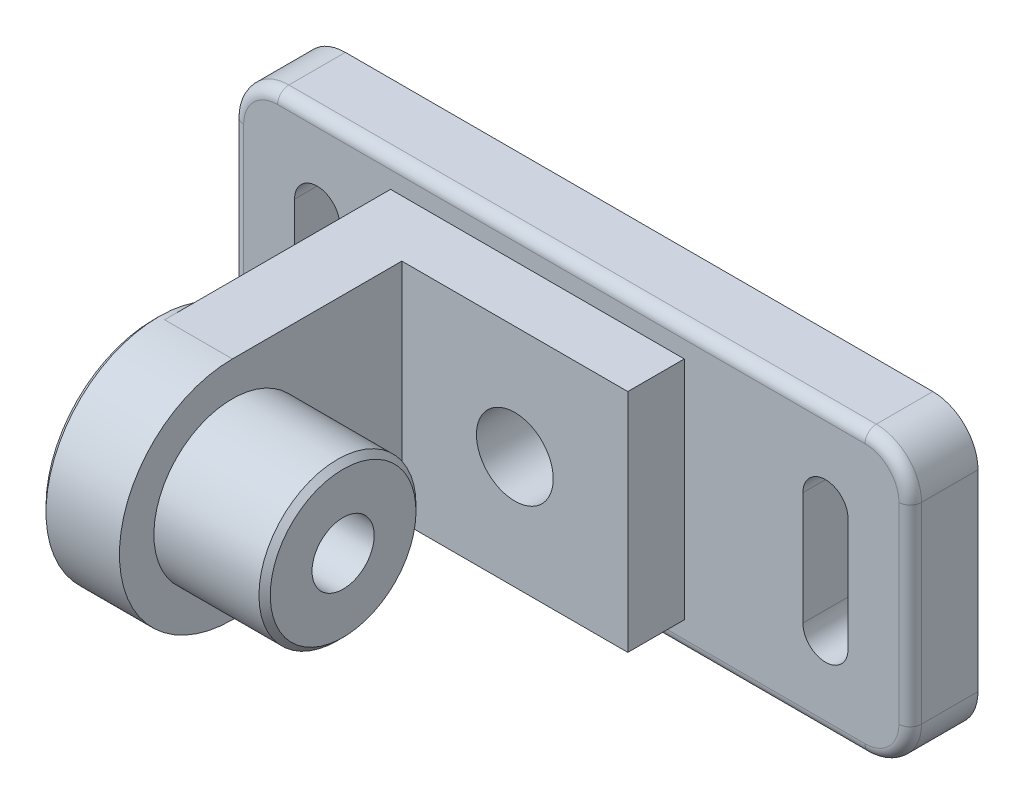
from build123d import *
from build123d.topology import SkipClean

# Parameters (mm, degrees)
SKETCH1_R               = 3.4
BOSS_EXTRUDE1_DEPTH     = 6
CHAMFER1_SIZE           = 1
SKETCH2_W               = 6
SKETCH2_H               = 20
BOSS_EXTRUDE2_DEPTH     = 30
CUT_EXTRUDE1_DEPTH      = 60.73483071
CUT_EXTRUDE1_DEPTH_BACK = 60.73483071
SKETCH3_R               = 2.75
SKETCH4_R               = 10
SKETCH4_R_2             = 2.75
BOSS_EXTRUDE3_DEPTH     = 1
CHAMFER2_SIZE           = 0.5
FILLET1_R               = 1
SKETCH5_W               = 20
SKETCH5_H               = 20
SKETCH5_R               = 3.4
BOSS_EXTRUDE4_DEPTH     = 5
CUT_EXTRUDE2_DEPTH      = 61.508263976
CUT_EXTRUDE2_DEPTH_BACK = 3
SKETCH7_R               = 6.95
SKETCH7_R_2             = 2.75
BOSS_EXTRUDE5_DEPTH     = 9.8
CHAMFER4_SIZE           = 0.5


with BuildPart() as part:
    # Sketch1 → Boss-Extrude1 (new body)
    with BuildSketch(Plane.XY):
        with BuildLine():
            Line((-26, 12.5), (26, 12.5))
            ThreePointArc((26, 12.5), (28.828427125, 11.328427125), (30, 8.5))
            Line((30, 8.5), (30, -8.5))
            ThreePointArc((30, -8.5), (28.828427125, -11.328427125), (26, -12.5))
            Line((26, -12.5), (-26, -12.5))
            ThreePointArc((-26, -12.5), (-28.828427125, -11.328427125), (-30, -8.5))
            Line((-30, -8.5), (-30, 8.5))
            ThreePointArc((-30, 8.5), (-28.828427125, 11.328427125), (-26, 12.5))
        make_face()
        Circle(SKETCH1_R, mode=Mode.SUBTRACT)
        with BuildLine():
            Line((-20.5, 5), (-20.5, -5))
            ThreePointArc((-20.5, -5), (-22.5, -7), (-24.5, -5))
            Line((-24.5, -5), (-24.5, 5))
            ThreePointArc((-24.5, 5), (-22.5, 7), (-20.5, 5))
        make_face(mode=Mode.SUBTRACT)
        with BuildLine():
            Line((20.5, 5), (20.5, -5))
            ThreePointArc((20.5, -5), (22.5, -7), (24.5, -5))
            Line((24.5, -5), (24.5, 5))
            ThreePointArc((24.5, 5), (22.5, 7), (20.5, 5))
        make_face(mode=Mode.SUBTRACT)
    extrude(amount=BOSS_EXTRUDE1_DEPTH)

    # Chamfer1
    chamfer1_edges = [part.edges().sort_by_distance(p)[0] for p in [
        (-3.4, 0, 0),
    ]]
    chamfer(chamfer1_edges, length=CHAMFER1_SIZE)

    # Sketch2 → Boss-Extrude2 (add)
    with BuildSketch(Plane.XY.offset(6)):
        with Locations((-13, 0)):
            Rectangle(SKETCH2_W, SKETCH2_H)
    extrude(amount=BOSS_EXTRUDE2_DEPTH)

    # Sketch3 → Cut-Extrude1 (cut, two sides: drawn at the far end of the back side and taken through both)
    with BuildSketch(Plane.ZY.offset(16).offset(-CUT_EXTRUDE1_DEPTH_BACK)):
        with Locations(Location((26, 0, 0), (0, 0, 270))):
            Circle(SKETCH3_R)
        with BuildLine():
            Line((26, 10), (26.394492089, 15.308450708))
            Line((26.394492089, 15.308450708), (43.333609146, 9.271325943))
            Line((43.333609146, 9.271325943), (37.706774414, -17.690590479))
            Line((37.706774414, -17.690590479), (26, -10))
            ThreePointArc((26, -10), (36, 0), (26, 10))
        make_face()
    extrude(amount=CUT_EXTRUDE1_DEPTH + CUT_EXTRUDE1_DEPTH_BACK, mode=Mode.SUBTRACT)

    # Sketch4 → Boss-Extrude3 (add, symmetric)
    with BuildSketch(Plane.ZY.offset(16)):
        with Locations(Location((26, 0, 0), (0, 0, 270))):
            Circle(SKETCH4_R)
        with Locations(Location((26, 0, 0), (0, 0, 270))):
            Circle(SKETCH4_R_2, mode=Mode.SUBTRACT)
    extrude(amount=BOSS_EXTRUDE3_DEPTH, both=True)

    # Chamfer2
    chamfer2_edges = [part.edges().sort_by_distance(p)[0] for p in [
        (-17, 10, 26),
    ]]
    chamfer(chamfer2_edges, length=CHAMFER2_SIZE)

    # Fillet1
    fillet1_edges = [part.edges().sort_by_distance(p)[0] for p in [
        (28.828427125, -11.328427125, 6),
        (30, 0, 6),
        (28.828427125, 11.328427125, 6),
        (0, 12.5, 6),
        (-28.828427125, 11.328427125, 6),
        (-30, 0, 6),
        (-28.828427125, -11.328427125, 6),
        (0, -12.5, 6),
    ]]
    fillet(fillet1_edges, radius=FILLET1_R)

    # Sketch5 → Boss-Extrude4 (add)
    with BuildSketch(Plane.XY.offset(6)):
        Rectangle(SKETCH5_W, SKETCH5_H)
        Circle(SKETCH5_R, mode=Mode.SUBTRACT)
    extrude(amount=BOSS_EXTRUDE4_DEPTH)

    # Sketch6 → Cut-Extrude2 (cut, two sides: drawn at the far end of the back side and taken through both)
    with BuildSketch(Plane.ZY.offset(17).offset(-CUT_EXTRUDE2_DEPTH_BACK)):
        Polygon((28.369738511, 4.098496398), (23.635467258, 4.10150195), (21.265728747, 0.003005552), (23.630261489, -4.098496398), (28.364532742, -4.10150195), (30.734271253, -0.003005552), align=None)
    extrude(amount=CUT_EXTRUDE2_DEPTH + CUT_EXTRUDE2_DEPTH_BACK, mode=Mode.SUBTRACT)

    # Sketch7 → Boss-Extrude5 (add)
    with SkipClean():  # the faces are left unmerged after this step: merging them gives an invalid solid
        with BuildSketch(Plane(origin=(-10, 0, 0), x_dir=(0, 0, -1), z_dir=(1, 0, 0))):
            with Locations(Location((-26, 0, 0), (0, 0, 270))):
                Circle(SKETCH7_R)
            with Locations(Location((-26, 0, 0), (0, 0, 180))):
                Circle(SKETCH7_R_2, mode=Mode.SUBTRACT)
        extrude(amount=BOSS_EXTRUDE5_DEPTH)

    # Chamfer4
    chamfer4_edges = [part.edges().sort_by_distance(p)[0] for p in [
        (-0.2, 6.95, 26),
    ]]
    chamfer(chamfer4_edges, length=CHAMFER4_SIZE)


solid = part.part
